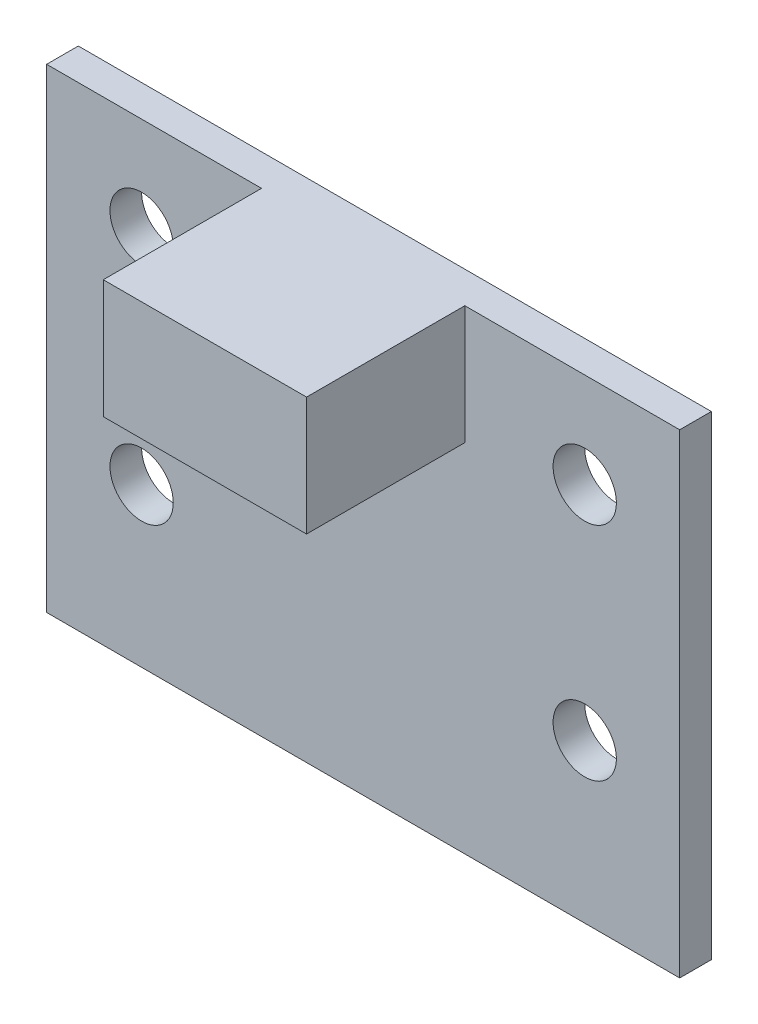
from build123d import *

# Parameters (mm, degrees)
SKETCH1_W           = 20
SKETCH1_H           = 15
SKETCH1_R           = 1
BOSS_EXTRUDE1_DEPTH = 1
SKETCH2_W           = 6.421944946
SKETCH2_H           = 3.747416962
BOSS_EXTRUDE2_DEPTH = 5


with BuildPart() as part:
    # Sketch1 → Boss-Extrude1 (new body)
    with BuildSketch(Plane.XY):
        Rectangle(SKETCH1_W, SKETCH1_H)
        with Locations((-7, 4.5)):
            Circle(SKETCH1_R, mode=Mode.SUBTRACT)
        with Locations((-7, -2.5)):
            Circle(SKETCH1_R, mode=Mode.SUBTRACT)
        with Locations((7, 4.5)):
            Circle(SKETCH1_R, mode=Mode.SUBTRACT)
        with Locations((7, -2.5)):
            Circle(SKETCH1_R, mode=Mode.SUBTRACT)
    extrude(amount=BOSS_EXTRUDE1_DEPTH)

    # Sketch2 → Boss-Extrude2 (add)
    with BuildSketch(Plane.XY.offset(1)):
        with Locations((0, 5.626291519)):
            Rectangle(SKETCH2_W, SKETCH2_H)
    extrude(amount=BOSS_EXTRUDE2_DEPTH)


solid = part.part
